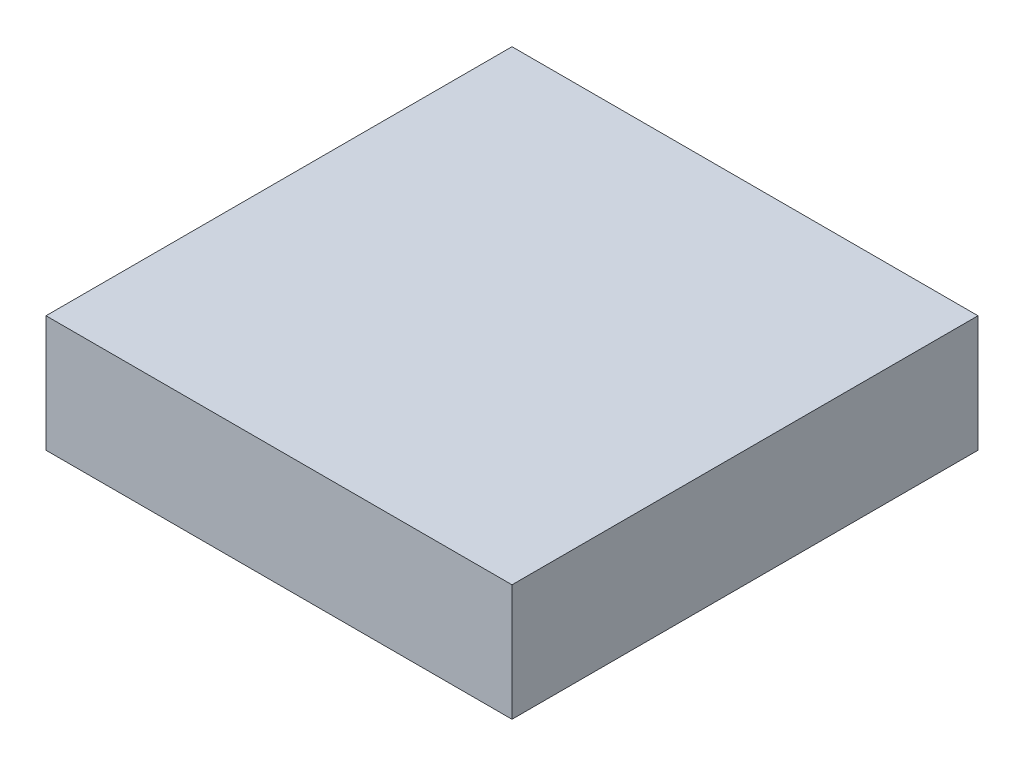
from build123d import *

# Parameters (mm, degrees)
SKETCH1_W           = 8
SKETCH1_H           = 8
BOSS_EXTRUDE1_DEPTH = 2


with BuildPart() as part:
    # Sketch1 → Boss-Extrude1 (new body)
    with BuildSketch(Plane(origin=(0, 0, 0), x_dir=(1, 0, 0), z_dir=(0, 1, 0))):
        Rectangle(SKETCH1_W, SKETCH1_H)
    extrude(amount=BOSS_EXTRUDE1_DEPTH)


solid = part.part
